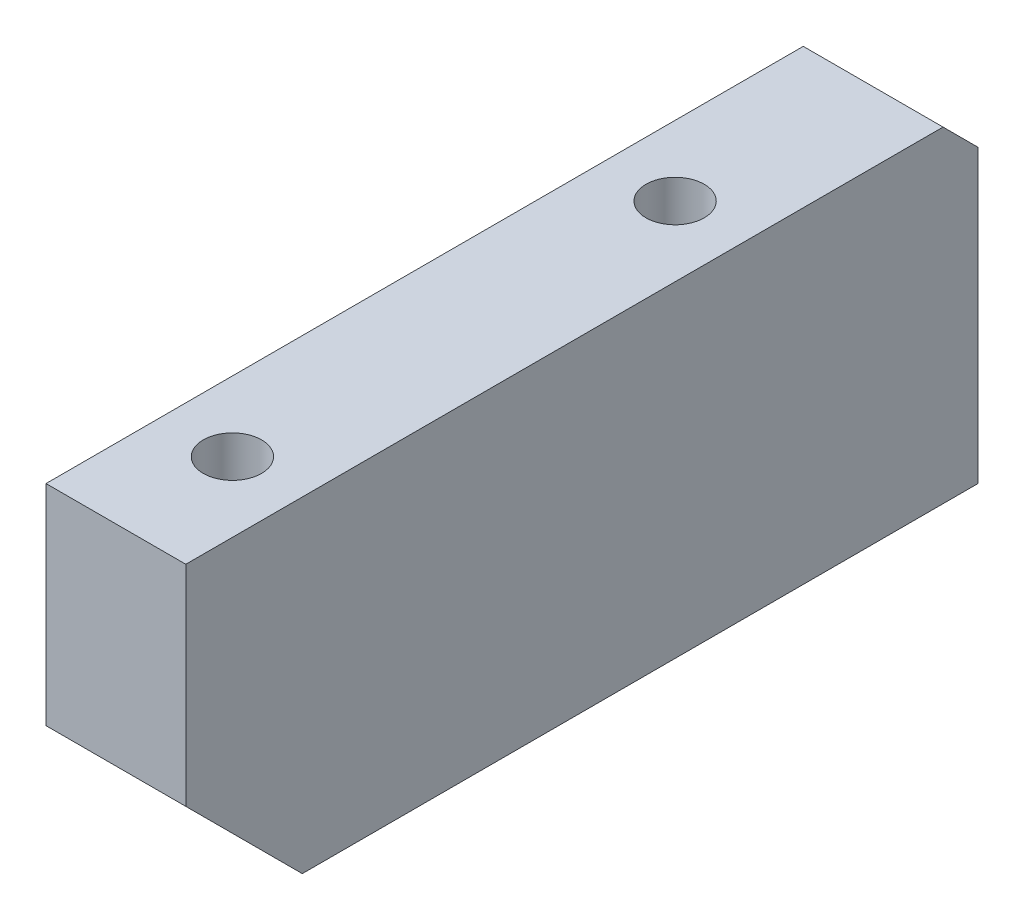
from build123d import *

# Parameters (mm, degrees)
SKETCH_1_W             = 12
SKETCH_1_H             = 28
EXTRUDE_1_DEPTH        = 68
CHAMFER_1_SIZE         = 10
CHAMFER_2_SIZE         = 3
HOLE_WIZARD_M6_1_D     = 5
HOLE_WIZARD_M6_1_DEPTH = 13
HOLE_WIZARD_M6_1_TIP   = 1.502151548
HOLE_WIZARD_M6_2_D     = 5
HOLE_WIZARD_M6_2_DEPTH = 13
HOLE_WIZARD_M6_2_TIP   = 1.502151548


with BuildPart() as part:
    # 草图1 → 凸台-拉伸1 (new body)
    with BuildSketch(Plane.XY):
        with Locations((-244.955728906, -14)):
            Rectangle(SKETCH_1_W, SKETCH_1_H)
    extrude(amount=EXTRUDE_1_DEPTH)

    # 倒角1
    chamfer_1_edges = [part.edges().sort_by_distance(p)[0] for p in [
        (-244.955728906, -28, 68),
    ]]
    chamfer(chamfer_1_edges, length=CHAMFER_1_SIZE)

    # 倒角2
    chamfer_2_edges = [part.edges().sort_by_distance(p)[0] for p in [
        (-244.955728906, 0, 0),
    ]]
    chamfer(chamfer_2_edges, length=CHAMFER_2_SIZE)

    # M6 螺纹孔1
    with Locations(Plane(origin=(0, 0, 0), x_dir=(-1, 0, 0), z_dir=(0, 0, -1))):
        with Locations((244.955728906, -9), (244.955728906, -21)):
            Hole(HOLE_WIZARD_M6_1_D / 2, depth=HOLE_WIZARD_M6_1_DEPTH)
            with Locations((0, 0, -(HOLE_WIZARD_M6_1_DEPTH + HOLE_WIZARD_M6_1_TIP / 2))):  # 118° drill point
                Cone(0, HOLE_WIZARD_M6_1_D / 2, HOLE_WIZARD_M6_1_TIP, mode=Mode.SUBTRACT)

    # M6 螺纹孔2
    with Locations(Plane(origin=(0, 0, 0), x_dir=(1, 0, 0), z_dir=(0, 1, 0))):
        with Locations((-244.955728906, -58), (-244.955728906, -20)):
            Hole(HOLE_WIZARD_M6_2_D / 2, depth=HOLE_WIZARD_M6_2_DEPTH)
            with Locations((0, 0, -(HOLE_WIZARD_M6_2_DEPTH + HOLE_WIZARD_M6_2_TIP / 2))):  # 118° drill point
                Cone(0, HOLE_WIZARD_M6_2_D / 2, HOLE_WIZARD_M6_2_TIP, mode=Mode.SUBTRACT)


solid = part.part
